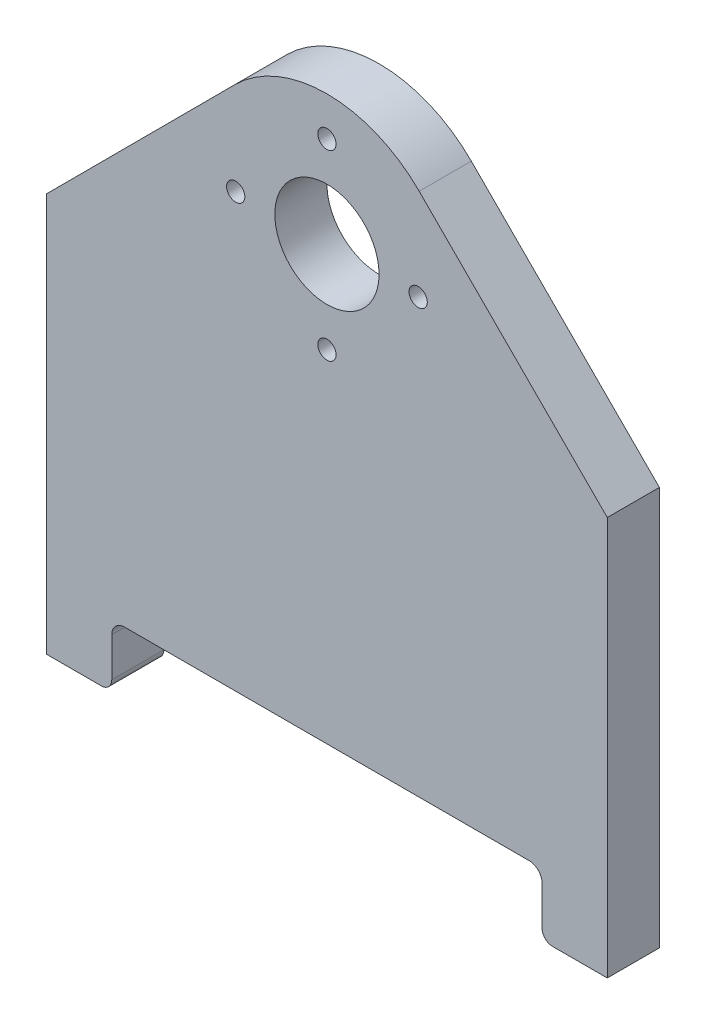
SolidWorks part; units mm, degrees
ref_plane "Front Plane" through (0, 0, 0) normal (0, 0, 1) x (1, 0, 0)
ref_plane "Top Plane" through (0, 0, 0) normal (0, 1, 0) x (1, 0, 0)
ref_plane "Right Plane" through (0, 0, 0) normal (1, 0, 0) x (0, 0, -1)
sketch "Sketch1" plane through (0, 0, 0) normal (0, 0, 1) x (1, 0, 0)
  line L0 (-215.1, -380) -> (-173.1, -380)
  line L1 (-215.1, -380) -> (-215.1, -74)
  line L2 (-215.1, -74) -> (-70.7893, 70.632)
  line L3 (215.1, -380) -> (215.1, -74)
  line L4 (215.1, -74) -> (70.7893, 70.632)
  line L5 (-155.1, -332) -> (155.1, -332)
  line L6 (-165.1, -342) -> (-165.1, -372)
  line L7 (165.1, -342) -> (165.1, -372)
  line L8 (173.1, -380) -> (215.1, -380)
  arc A0 (70.7893, 70.632) -> (-70.7893, 70.632) centre (0, 0) ccw
  arc A1 (165.1, -372) -> (173.1, -380) centre (173.1, -372) ccw
  arc A2 (-165.1, -372) -> (-173.1, -380) centre (-173.1, -372) cw
  arc A3 (155.1, -332) -> (165.1, -342) centre (155.1, -342) cw
  arc A4 (-165.1, -342) -> (-155.1, -332) centre (-155.1, -342) cw
  circle A6 centre (0, 0) radius 40
  dimension "D1" = 200
  dimension "D10" = 8
  dimension "D11" = 8
  dimension "D12" = 10
  dimension "D13" = 10
  dimension "D14" = 80
  dimension "D2" = 380
  dimension "D3" = 215.1
  dimension "D4" = 430.2
  dimension "D5" = 306
  dimension "D6" = 306
  dimension "D7" = 48
  dimension "D8" = 50
  dimension "D9" = 50
extrude "Boss-Extrude1" add sketch "Sketch1" along normal blind 40
hole_wizard "M16 Tapped Hole1" positions "Sketch3" profile "Sketch4" tap size "M16" standard "GB" end condition through all
sketch "Sketch3" plane through (0, 0, 40) normal (0, 0, 1) x (1, 0, 0)
  circle A0 centre (0, 0) radius 70 construction
  point P0 (0, 70)
  point P25 (70, 0)
  point P26 (0, -70)
  point P27 (-70, 0)
  dimension "D1" = 140
  dimension "D2" = 4
sketch "Sketch4" plane through (0, 70, 40) normal (1, 0, 0) x (0, -1, 0)
  line L0 (0, 0) -> (0, 40)
  line L1 (0, 40) -> (7, 40)
  line L2 (7, 40) -> (7, 0)
  line L5 (7, 0) -> (0, 0)
  line L11 (0, -6.35) -> (0, 107.95) construction
  dimension "通孔螺纹孔钻头直径" = 14
  dimension "通孔螺纹孔钻头深度" = 40
cosmetic thread "CosmeticThread hole thread 1" parameters "D2"=16
cosmetic thread "CosmeticThread hole thread 2" parameters "D2"=16
cosmetic thread "CosmeticThread hole thread 3" parameters "D2"=16
cosmetic thread "CosmeticThread hole thread 4" parameters "D2"=16
